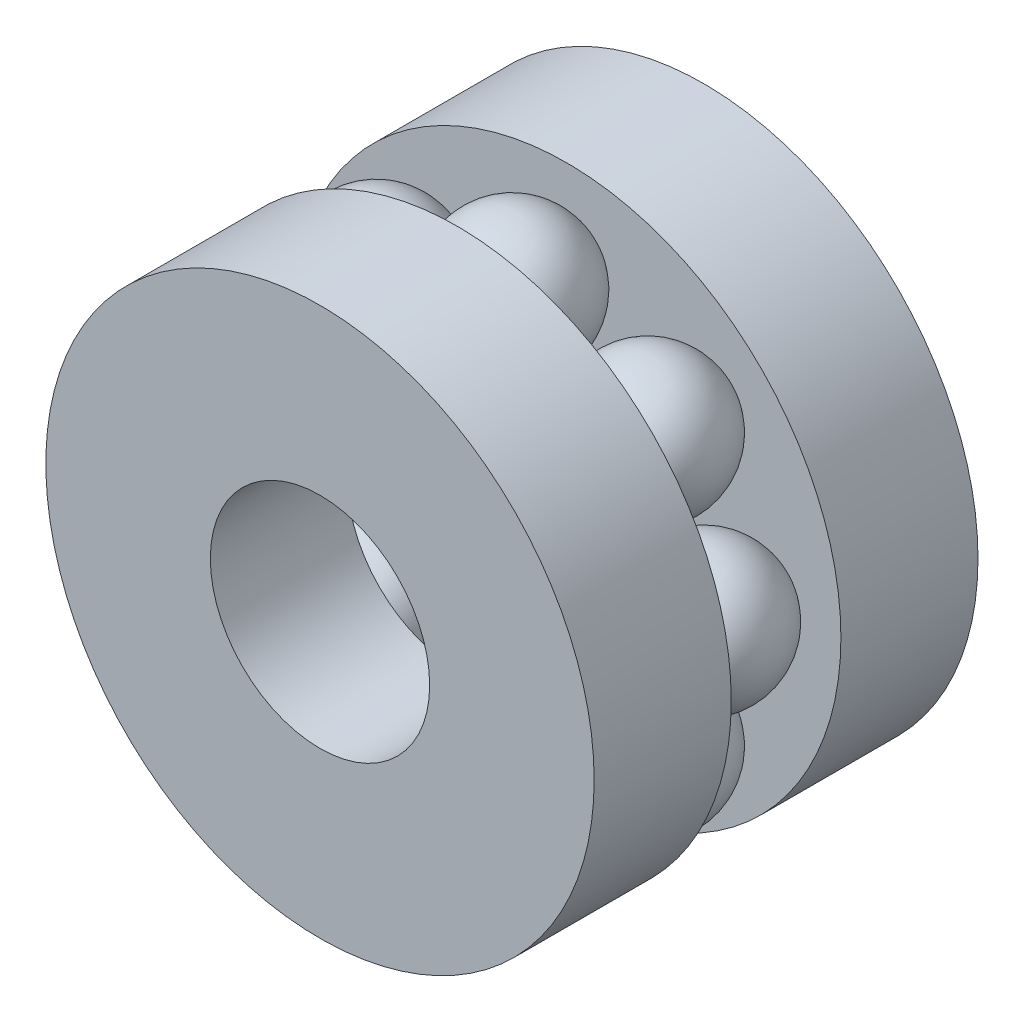
from build123d import *

# Parameters (mm, degrees)
BOSS_EXTRUDE1_START = 5
SKETCH1_R           = 10
SKETCH1_R_2         = 4
BOSS_EXTRUDE1_DEPTH = 5
CIRPATTERN2_COUNT   = 8
BOSS_EXTRUDE2_START = -4
SKETCH3_R           = 10
SKETCH3_R_2         = 4
BOSS_EXTRUDE2_DEPTH = 5


with BuildPart() as part:
    # Sketch1 → Boss-Extrude1 (new body)
    with BuildSketch(Plane.XY.offset(BOSS_EXTRUDE1_START)):
        Circle(SKETCH1_R)
        Circle(SKETCH1_R_2, mode=Mode.SUBTRACT)
    extrude(amount=BOSS_EXTRUDE1_DEPTH)

    # Sketch2 → Revolve1 (revolve)
    with BuildSketch(Plane(origin=(0, 0, 0), x_dir=(0, 0, -1), z_dir=(1, 0, 0))):
        with BuildLine():
            Line((-3, 4.5), (-3, 9.5))
            ThreePointArc((-3, 9.5), (-5.5, 7), (-3, 4.5))
        make_face()
    revolve1 = revolve(axis=Axis((0, 4.5, 3), (0, 1, 0)))

    # CirPattern2: Revolve1 ×8 about axis
    cirpattern2_axis = Axis((0, 0, 0), (0, 0, 1))
    for i in range(1, CIRPATTERN2_COUNT):
        add(revolve1.rotate(cirpattern2_axis, i * 360 / CIRPATTERN2_COUNT))

    # Sketch3 → Boss-Extrude2 (add)
    with BuildSketch(Plane.XY.offset(BOSS_EXTRUDE2_START)):
        Circle(SKETCH3_R)
        Circle(SKETCH3_R_2, mode=Mode.SUBTRACT)
    extrude(amount=BOSS_EXTRUDE2_DEPTH)


solid = part.part
